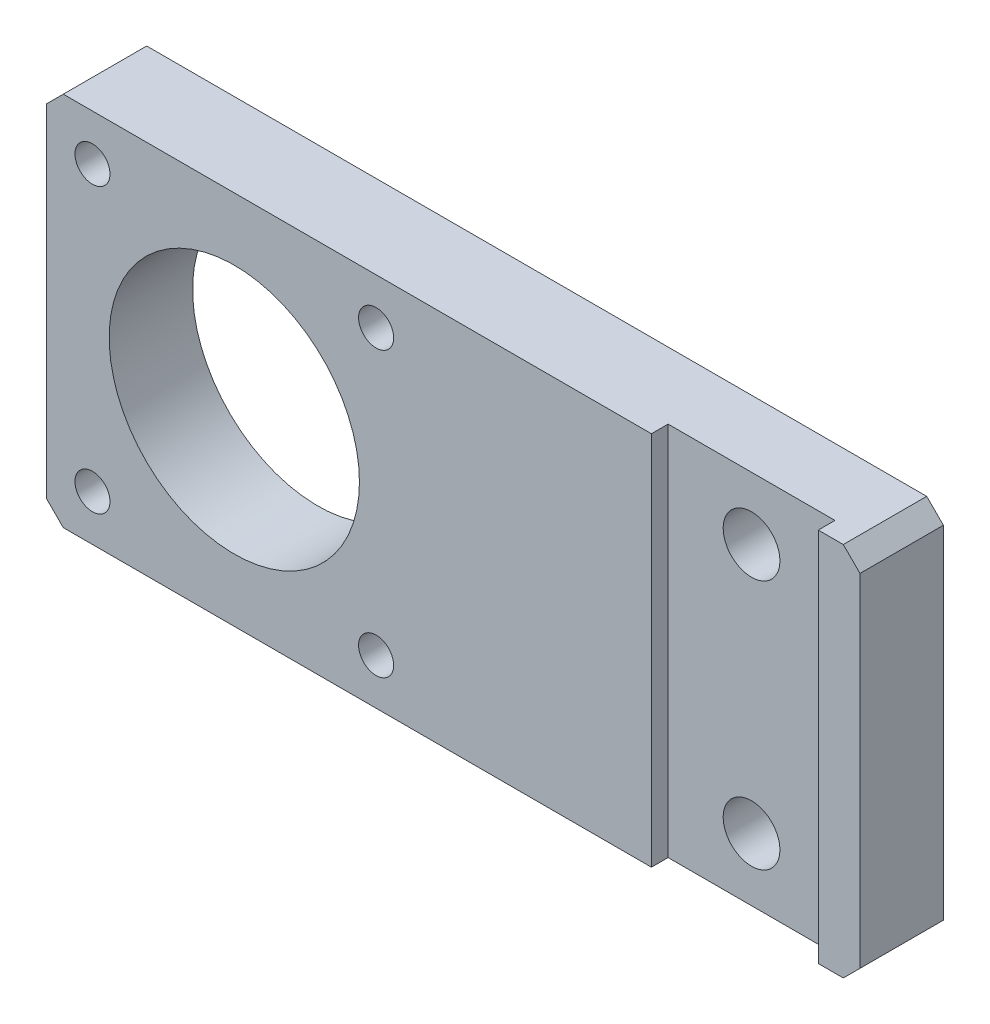
from build123d import *

# Parameters (mm, degrees)
SKETCH1_W             = 97.5
SKETCH1_H             = 45
SKETCH1_R             = 15
SKETCH1_R_2           = 3.4
BOSS_EXTRUDE1_DEPTH   = 10
CUT_EXTRUDE1_REACH    = 109.848
SKETCH2_W             = 20
SKETCH2_H             = 2
M5_TAPPED_HOLE1_D     = 4.2
M5_TAPPED_HOLE1_DEPTH = 12.4
M5_TAPPED_HOLE1_TIP   = 1.2618073
CHAMFER1_SIZE         = 2


with BuildPart() as part:
    # Sketch1 → Boss-Extrude1 (new body)
    with BuildSketch(Plane.XY):
        with Locations((48.75, 22.5)):
            Rectangle(SKETCH1_W, SKETCH1_H)
        with Locations((22.5, 22.5)):
            Circle(SKETCH1_R, mode=Mode.SUBTRACT)
        with Locations((82.5, 37.5)):
            Circle(SKETCH1_R_2, mode=Mode.SUBTRACT)
        with Locations((82.5, 7.5)):
            Circle(SKETCH1_R_2, mode=Mode.SUBTRACT)
    extrude(amount=BOSS_EXTRUDE1_DEPTH)

    # Sketch2 → Cut-Extrude1 (cut, up to next)
    with BuildSketch(Plane(origin=(0, 45, 0), x_dir=(1, 0, 0), z_dir=(0, 1, 0)), mode=Mode.PRIVATE) as cut_extrude1_sk1:
        with Locations((82.5, -9)):
            Rectangle(SKETCH2_W, SKETCH2_H)
    cut_extrude1_tool1 = extrude(cut_extrude1_sk1.sketch, amount=-CUT_EXTRUDE1_REACH, mode=Mode.PRIVATE) & part.part
    add(cut_extrude1_tool1.solids().sort_by_distance((82.5, 45, 9))[0], mode=Mode.SUBTRACT)

    # M5 Tapped Hole1
    with Locations(Plane(origin=(0, 0, 0), x_dir=(-1, 0, 0), z_dir=(0, 0, -1))):
        with Locations((-39.5, 5.5), (-5.5, 5.5), (-5.5, 39.5), (-39.5, 39.5)):
            Hole(M5_TAPPED_HOLE1_D / 2, depth=M5_TAPPED_HOLE1_DEPTH)
            with Locations((0, 0, -(M5_TAPPED_HOLE1_DEPTH + M5_TAPPED_HOLE1_TIP / 2))):  # 118° drill point
                Cone(0, M5_TAPPED_HOLE1_D / 2, M5_TAPPED_HOLE1_TIP, mode=Mode.SUBTRACT)

    # Chamfer1
    chamfer1_edges = [part.edges().sort_by_distance(p)[0] for p in [
        (0, 45, 5),
        (97.5, 45, 5),
        (97.5, 0, 5),
        (0, 0, 5),
    ]]
    chamfer(chamfer1_edges, length=CHAMFER1_SIZE)


solid = part.part
